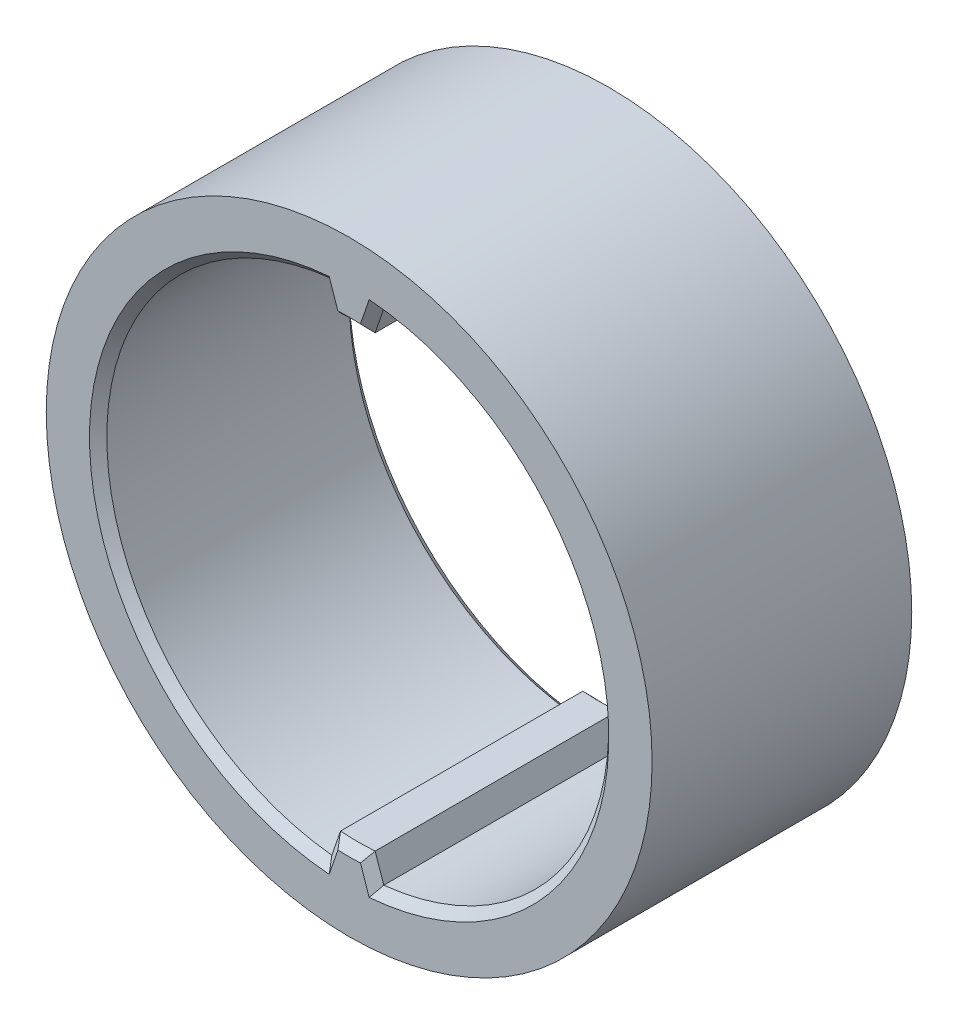
from build123d import *

# Parameters (mm, degrees)
SKETCH2_R           = 17.5
SKETCH2_R_2         = 14.5
BOSS_EXTRUDE1_DEPTH = 15
BOSS_EXTRUDE2_DEPTH = 15
CHAMFER1_SIZE       = 0.5


with BuildPart() as part:
    # Sketch2 → Boss-Extrude1 (new body)
    with BuildSketch(Plane.XY):
        Circle(SKETCH2_R)
        Circle(SKETCH2_R_2, mode=Mode.SUBTRACT)
    extrude(amount=BOSS_EXTRUDE1_DEPTH)

    # Sketch4 → Boss-Extrude2 (add)
    with BuildSketch(Plane.XY):
        with BuildLine():
            Line((-1.5, 14.422205102), (-1, 12.961481397))
            ThreePointArc((-1, 12.961481397), (0, 13), (1, 12.961481397))
            Line((1, 12.961481397), (1.5, 14.422205102))
            ThreePointArc((1.5, 14.422205102), (0, 14.5), (-1.5, 14.422205102))
        make_face()
        with BuildLine():
            Line((1, -12.961481397), (1.5, -14.422205102))
            ThreePointArc((1.5, -14.422205102), (0, -14.5), (-1.5, -14.422205102))
            Line((-1.5, -14.422205102), (-1, -12.961481397))
            ThreePointArc((-1, -12.961481397), (0, -13), (1, -12.961481397))
        make_face()
    extrude(amount=BOSS_EXTRUDE2_DEPTH)

    # Chamfer1
    chamfer1_edges = [part.edges().sort_by_distance(p)[0] for p in [
        (-14.5, 0, 15),
        (-14.5, 0, 0),
        (-1.25, 13.691843249, 0),
        (0, 13, 0),
        (1.25, 13.691843249, 0),
        (1.25, 13.691843249, 15),
        (-1.25, 13.691843249, 15),
        (0, 13, 15),
        (14.5, 0, 0),
        (14.5, 0, 15),
        (1.25, -13.691843249, 0),
        (0, -13, 0),
        (-1.25, -13.691843249, 0),
        (-1.25, -13.691843249, 15),
        (1.25, -13.691843249, 15),
        (0, -13, 15),
    ]]
    chamfer(chamfer1_edges, length=CHAMFER1_SIZE)


solid = part.part
